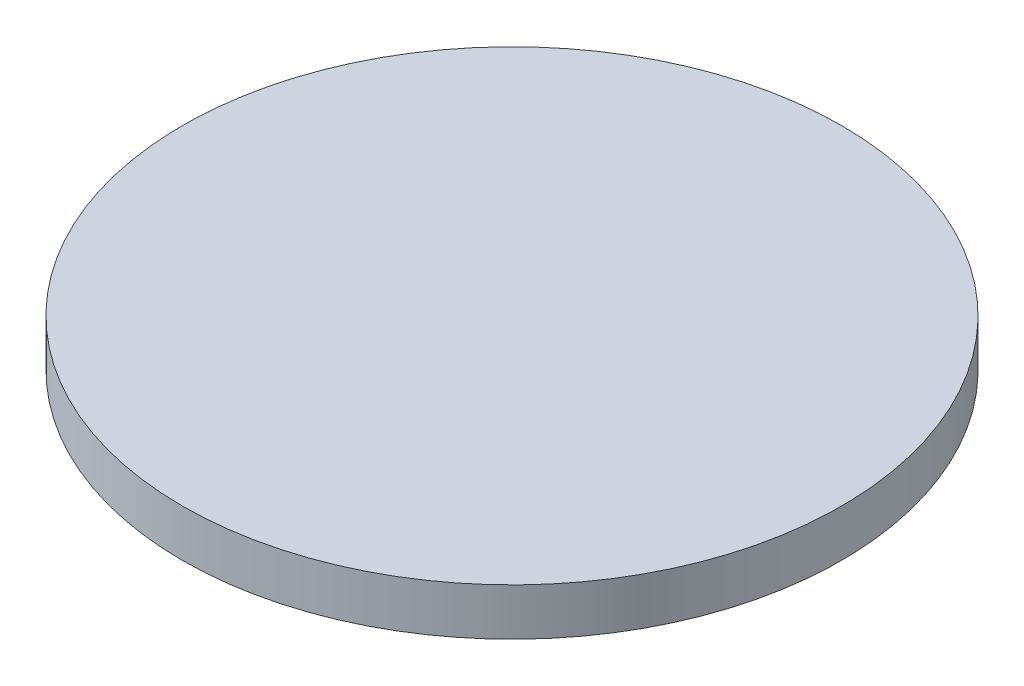
SolidWorks part; units mm, degrees
material "成品"
ref_plane "Front Plane" through (0, 0, 0) normal (0, 0, 1) x (1, 0, 0)
ref_plane "Top Plane" through (0, 0, 0) normal (0, 1, 0) x (1, 0, 0)
ref_plane "Right Plane" through (0, 0, 0) normal (1, 0, 0) x (0, 0, -1)
sketch "Sketch1" plane through (0, 0, 0) normal (0, 1, 0) x (1, 0, 0)
  circle A0 centre (0, 0) radius 14
  dimension "D1" = 28
extrude "Boss-Extrude1" add sketch "Sketch1" along normal blind 2
